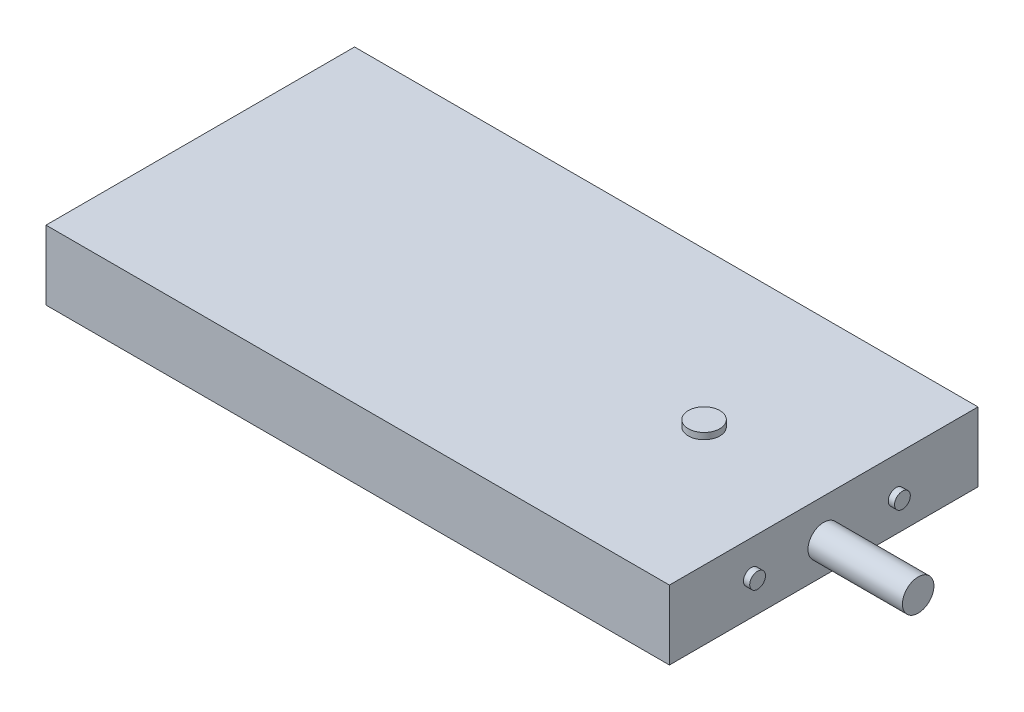
from build123d import *

# Parameters (mm, degrees)
SKETCH1_W           = 198
SKETCH1_H           = 98
BOSS_EXTRUDE1_DEPTH = 22
SKETCH2_R           = 5
BOSS_EXTRUDE2_DEPTH = 30
SKETCH3_R           = 5
BOSS_EXTRUDE3_DEPTH = 2
SKETCH4_R           = 2.5
BOSS_EXTRUDE4_DEPTH = 2


with BuildPart() as part:
    # Sketch1 → Boss-Extrude1 (new body)
    with BuildSketch(Plane(origin=(0, 0, 0), x_dir=(1, 0, 0), z_dir=(0, 1, 0))):
        Rectangle(SKETCH1_W, SKETCH1_H)
    extrude(amount=BOSS_EXTRUDE1_DEPTH)

    # Sketch2 → Boss-Extrude2 (add)
    with BuildSketch(Plane(origin=(99, 0, 0), x_dir=(0, 0, -1), z_dir=(1, 0, 0))):
        with Locations(Location((0, 9.760048185, 0), (0, 0, 180))):
            Circle(SKETCH2_R)
    extrude(amount=BOSS_EXTRUDE2_DEPTH)

    # Sketch3 → Boss-Extrude3 (add)
    with BuildSketch(Plane(origin=(0, 22, 0), x_dir=(1, 0, 0), z_dir=(0, 1, 0))):
        with Locations(Location((61, 0, 0), (0, 0, 90))):
            Circle(SKETCH3_R)
    extrude(amount=BOSS_EXTRUDE3_DEPTH)

    # Sketch4 → Boss-Extrude4 (add)
    with BuildSketch(Plane(origin=(99, 0, 0), x_dir=(0, 0, -1), z_dir=(1, 0, 0))):
        with Locations(Location((23, 10.330807158, 0), (0, 0, 180))):
            Circle(SKETCH4_R)
        with Locations(Location((-23, 11.325219915, 0), (0, 0, 180))):
            Circle(SKETCH4_R)
    extrude(amount=BOSS_EXTRUDE4_DEPTH)


solid = part.part
